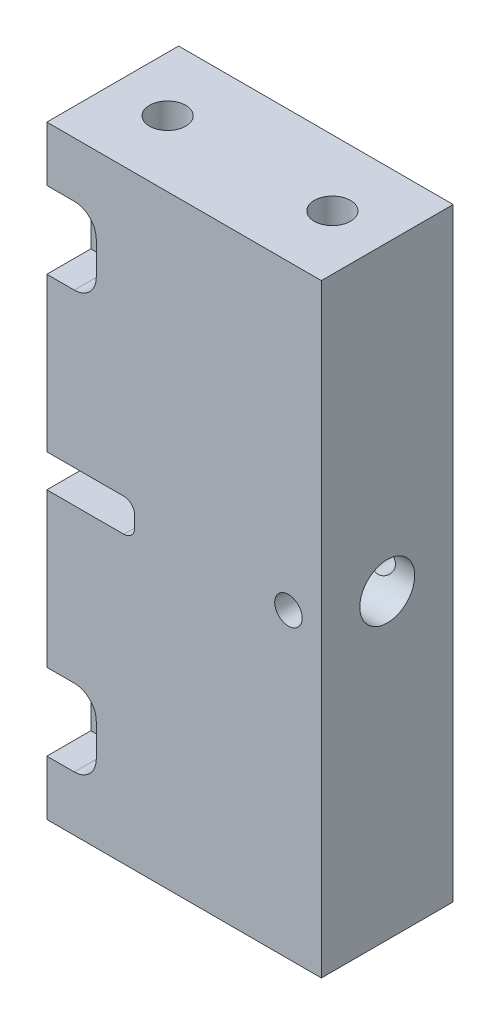
from build123d import *

# Parameters (mm, degrees)
SKETCH_1_W                  = 12
SKETCH_1_H                  = 55
EXTRUDE_1_DEPTH             = 25
SKETCH_2_R                  = 1.1
CUT_EXTRUDE_1_DEPTH         = 25
SKETCH_3_R                  = 2.5
CUT_EXTRUDE_2_DEPTH         = 8
SKETCH_4_W                  = 16
SKETCH_4_H                  = 3
CUT_EXTRUDE_3_DEPTH         = 6
HOLE_WIZARD_M4_1_AT_2_COUNT = 2
HOLE_WIZARD_M4_1_AT_2_PITCH = 15
FILLET_1_R                  = 1
CUT_EXTRUDE_4_DEPTH         = 4
HOLE_WIZARD_M3_1_D          = 2.5
FILLET_2_R                  = 1


with BuildPart() as part:
    # 草图1 → 凸台-拉伸1 (new body)
    with BuildSketch(Plane(origin=(0, 0, 0), x_dir=(0, 0, -1), z_dir=(1, 0, 0))):
        Rectangle(SKETCH_1_W, SKETCH_1_H)
    extrude(amount=EXTRUDE_1_DEPTH)

    # 草图2 → 切除-拉伸1 (cut)
    with BuildSketch(Plane(origin=(25, 0, 0), x_dir=(0, 0, -1), z_dir=(1, 0, 0))):
        Circle(SKETCH_2_R)
    extrude(amount=-CUT_EXTRUDE_1_DEPTH, mode=Mode.SUBTRACT)

    # 草图3 → 切除-拉伸2 (cut)
    with BuildSketch(Plane(origin=(25, 0, 0), x_dir=(0, 0, -1), z_dir=(1, 0, 0))):
        Circle(SKETCH_3_R)
    extrude(amount=-CUT_EXTRUDE_2_DEPTH, mode=Mode.SUBTRACT)

    # 草图4 → 切除-拉伸3 (cut)
    with BuildSketch(Plane.XY.offset(6)):
        Rectangle(SKETCH_4_W, SKETCH_4_H)
    extrude(amount=-CUT_EXTRUDE_3_DEPTH, mode=Mode.SUBTRACT)

    # 草图7 → M4 螺纹孔1 (revolve, cut)
    with BuildSketch(Plane(origin=(5, 27.5, 0), x_dir=(0, 0, 1), z_dir=(1, 0, 0))):
        Polygon((0, 0), (0, 11.091420021), (1.65, 10.1), (1.65, 0), align=None)
    hole_wizard_m4_1 = revolve(axis=Axis((5, 33.85, 0), (0, -1, 0)), mode=Mode.SUBTRACT)

    # M4 螺纹孔1 at 2: M4 螺纹孔1 ×2
    with Locations(*[(i * HOLE_WIZARD_M4_1_AT_2_PITCH, 0, 0) for i in range(1, HOLE_WIZARD_M4_1_AT_2_COUNT)]):
        add(hole_wizard_m4_1, mode=Mode.SUBTRACT)

    # 镜向1: M4 螺纹孔1 across plane
    add(hole_wizard_m4_1.mirror(Plane.ZX), mode=Mode.SUBTRACT)

    # 镜向1 copy 1 sketch → 镜向1 copy 1 (revolve, cut)
    with BuildSketch(Plane(origin=(20, -27.5, 0), x_dir=(0, 0, 1), z_dir=(1, 0, 0))):
        Polygon((0, 0), (0, -11.091420021), (1.65, -10.1), (1.65, 0), align=None)
    revolve(axis=Axis((20, -33.85, 0), (0, -1, 0)), mode=Mode.SUBTRACT)

    # 圆角1
    fillet_1_edges = [part.edges().sort_by_distance(p)[0] for p in [
        (8, -1.5, 3),
        (8, 1.5, 3),
    ]]
    fillet(fillet_1_edges, radius=FILLET_1_R)

    # 草图9 → 切除-拉伸4 (cut)
    with BuildSketch(Plane.XY.offset(6)):
        with BuildLine():
            Line((-4.5, 22.5), (2.5, 22.5))
            ThreePointArc((2.5, 22.5), (3.914213562, 21.914213562), (4.5, 20.5))
            Line((4.5, 20.5), (4.5, 17.5))
            ThreePointArc((4.5, 17.5), (3.914213562, 16.085786438), (2.5, 15.5))
            Line((2.5, 15.5), (-4.5, 15.5))
            Line((-4.5, 15.5), (-4.5, 22.5))
        make_face()
    cut_extrude_4 = extrude(amount=-CUT_EXTRUDE_4_DEPTH, mode=Mode.SUBTRACT)

    # 镜向2: 切除-拉伸4 across plane
    add(cut_extrude_4.mirror(Plane.ZX), mode=Mode.SUBTRACT)

    # M3 螺纹孔1 (through all)
    with Locations(Plane.XY.offset(6)):
        with Locations((22, 0)):
            Hole(HOLE_WIZARD_M3_1_D / 2)

    # 圆角2
    fillet_2_edges = [part.edges().sort_by_distance(p)[0] for p in [
        (17, 0, 1.1),
    ]]
    fillet(fillet_2_edges, radius=FILLET_2_R)


solid = part.part
